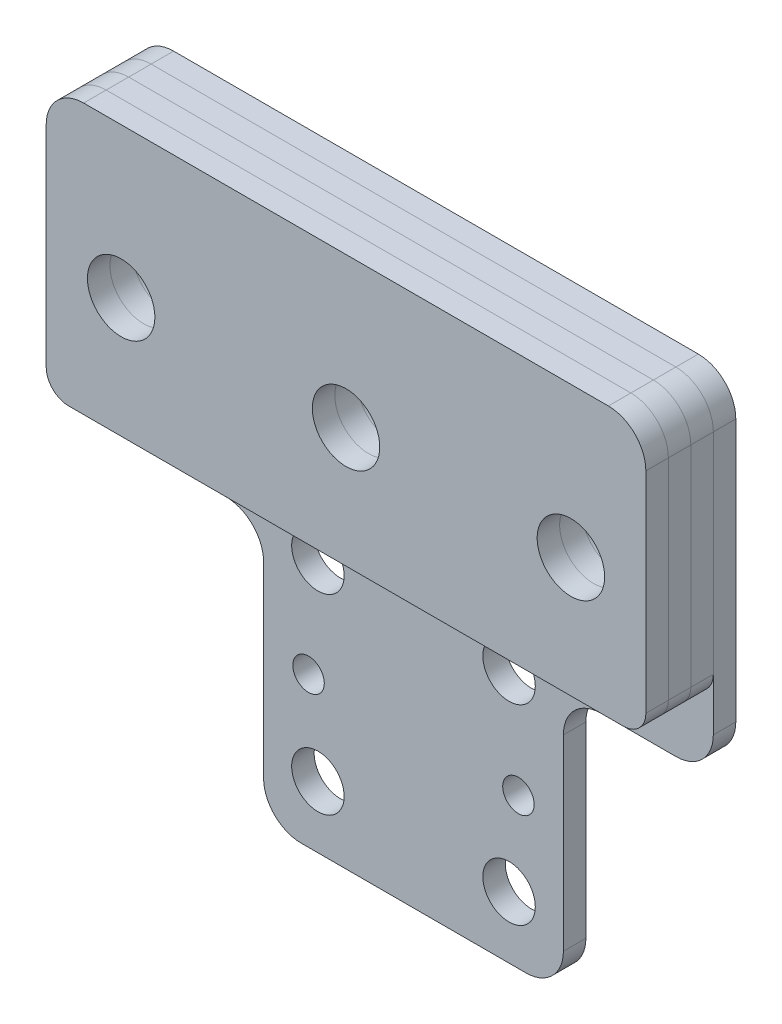
from build123d import *

# Parameters (mm, degrees)
SKETCH_1_W             = 80
SKETCH_1_H             = 80
EXTRUDE_1_DEPTH        = 3
SKETCH_5_W             = 20
SKETCH_5_H             = 35
CUT_EXTRUDE_3_DEPTH    = 3
FILLET_1_R             = 5
SKETCH_2_R             = 4.5
CUT_EXTRUDE_1_DEPTH    = 3
SKETCH_3_R             = 3.5
CUT_EXTRUDE_2_DEPTH    = 3
SKETCH_4_R             = 4.5
EXTRUDE_2_DEPTH        = 3
FILLET_2_R             = 3
PATTERN_LINEAR_1_COUNT = 3
PATTERN_LINEAR_1_PITCH = 3
SKETCH_6_R             = 2.1
CUT_EXTRUDE_4_DEPTH    = 3
FILLET_3_R             = 5


with BuildPart() as part:
    # 草图1 → 凸台-拉伸1 (new body)
    with BuildSketch(Plane.XY):
        Rectangle(SKETCH_1_W, SKETCH_1_H)
    extrude(amount=EXTRUDE_1_DEPTH)

    # 草图5 → 切除-拉伸3 (cut)
    with BuildSketch(Plane.XY.offset(3)):
        with Locations((30, -22.5)):
            Rectangle(SKETCH_5_W, SKETCH_5_H)
        with Locations((-30, -22.5)):
            Rectangle(SKETCH_5_W, SKETCH_5_H)
    extrude(amount=-CUT_EXTRUDE_3_DEPTH, mode=Mode.SUBTRACT)

    # 圆角1
    fillet_1_edges = [part.edges().sort_by_distance(p)[0] for p in [
        (40, -5, 1.5),
        (20, -40, 1.5),
        (-20, -40, 1.5),
        (-40, -5, 1.5),
        (-40, 40, 1.5),
        (40, 40, 1.5),
    ]]
    fillet(fillet_1_edges, radius=FILLET_1_R)

    # 草图2 → 切除-拉伸1 (cut)
    with BuildSketch(Plane.XY.offset(3)):
        with Locations((-30, 20)):
            Circle(SKETCH_2_R)
        with Locations((0, 20)):
            Circle(SKETCH_2_R)
        with Locations((30, 20)):
            Circle(SKETCH_2_R)
    extrude(amount=-CUT_EXTRUDE_1_DEPTH, mode=Mode.SUBTRACT)

    # 草图3 → 切除-拉伸2 (cut)
    with BuildSketch(Plane.XY.offset(3)):
        with Locations((12.75, -6.25)):
            Circle(SKETCH_3_R)
        with Locations((12.75, -31.75)):
            Circle(SKETCH_3_R)
        with Locations((-12.75, -31.75)):
            Circle(SKETCH_3_R)
        with Locations((-12.75, -6.25)):
            Circle(SKETCH_3_R)
    extrude(amount=-CUT_EXTRUDE_2_DEPTH, mode=Mode.SUBTRACT)

    # 草图6 → 切除-拉伸4 (cut)
    with BuildSketch(Plane(origin=(0, 0, 0), x_dir=(-1, 0, 0), z_dir=(0, 0, -1))):
        with Locations((-14, -20)):
            Circle(SKETCH_6_R)
        with Locations(Location((14, -20, 0), (0, 0, 180))):
            Circle(SKETCH_6_R)
    extrude(amount=-CUT_EXTRUDE_4_DEPTH, mode=Mode.SUBTRACT)

    # 圆角3
    fillet_3_edges = [part.edges().sort_by_distance(p)[0] for p in [
        (20, -5, 1.5),
        (-20, -5, 1.5),
    ]]
    fillet(fillet_3_edges, radius=FILLET_3_R)


with BuildPart() as body_2:
    # 草图4 → 凸台-拉伸2 (new body)
    with BuildSketch(Plane.XY.offset(3)):
        with BuildLine():
            Line((-40, 4), (40, 4))
            Line((40, 4), (40, 35))
            ThreePointArc((40, 35), (38.535533906, 38.535533906), (35, 40))
            Line((35, 40), (-35, 40))
            ThreePointArc((-35, 40), (-38.535533906, 38.535533906), (-40, 35))
            Line((-40, 35), (-40, 4))
        make_face()
        with Locations((30, 20)):
            Circle(SKETCH_4_R, mode=Mode.SUBTRACT)
        with Locations((-30, 20)):
            Circle(SKETCH_4_R, mode=Mode.SUBTRACT)
        with Locations((0, 20)):
            Circle(SKETCH_4_R, mode=Mode.SUBTRACT)
    extrude(amount=EXTRUDE_2_DEPTH)

    # 圆角2
    fillet_2_edges = [body_2.edges().sort_by_distance(p)[0] for p in [
        (40, 4, 4.5),
        (-40, 4, 4.5),
    ]]
    fillet(fillet_2_edges, radius=FILLET_2_R)


with BuildPart() as pattern_linear_1_1:
    # 阵列(线性)1: pattern copy
    add(body_2.part.moved(Location(Vector(0, 0, 1) * (1 * PATTERN_LINEAR_1_PITCH))))


with BuildPart() as pattern_linear_1_2:
    # 阵列(线性)1: pattern copy
    add(body_2.part.moved(Location(Vector(0, 0, 1) * (2 * PATTERN_LINEAR_1_PITCH))))


solid = Compound([part.part, body_2.part, pattern_linear_1_1.part, pattern_linear_1_2.part])
